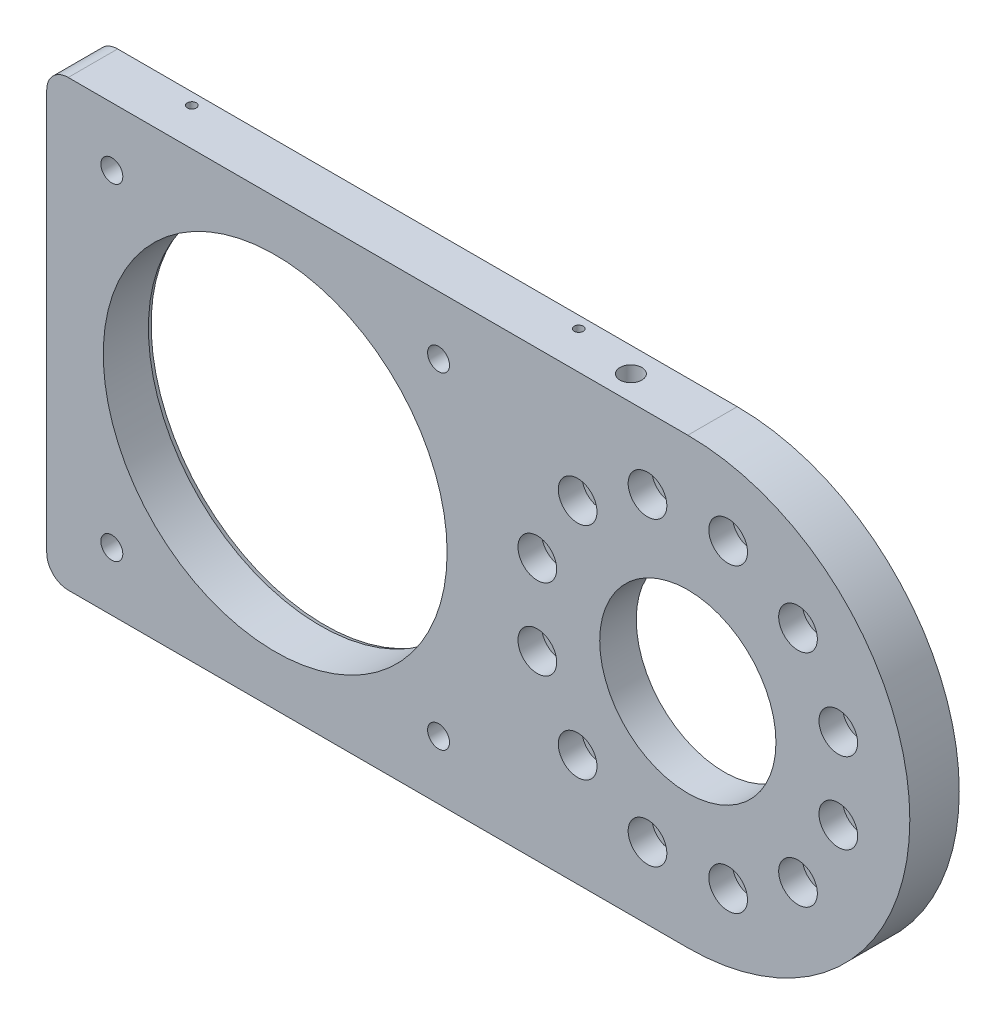
from build123d import *

# Parameters (mm, degrees)
BOSS_EXTRUDE1_DEPTH                                  = 23
FILLET1_R                                            = 10
HOLE_SIZE_PER_SOCKET_HEAD_CAP_SCREW_TYPE_D           = 11
HOLE_SIZE_PER_SOCKET_HEAD_CAP_SCREW_TYPE_CBORE_D     = 18
HOLE_SIZE_PER_SOCKET_HEAD_CAP_SCREW_TYPE_CBORE_DEPTH = 11
CIRPATTERN1_COUNT                                    = 12
SKETCH8_R                                            = 80
CUT_EXTRUDE1_DEPTH                                   = 23
SKETCH13_R                                           = 41
CUT_EXTRUDE3_DEPTH                                   = 23
SKETCH14_R                                           = 57.5
CUT_EXTRUDE4_DEPTH                                   = 6
M12_TAPPED_HOLE2_D                                   = 10.2
M5_TAPPED_HOLE1_AT_2_COUNT                           = 2
M5_TAPPED_HOLE1_AT_2_PITCH                           = 180
CHAMFER3_SIZE                                        = 2
CHAMFER3_SIZE2                                       = 0.727940469
CHAMFER4_SIZE                                        = 2
CHAMFER4_SIZE2                                       = 0.727940469
M5_TAPPED_HOLE3_D                                    = 4.2
M5_TAPPED_HOLE3_DEPTH                                = 12.4
M5_TAPPED_HOLE3_TIP                                  = 1.2618073


with BuildPart() as part:
    # Sketch1 → Boss-Extrude1 (new body)
    with BuildSketch(Plane.XY):
        with BuildLine():
            Line((0, 0), (298.3, 0))
            ThreePointArc((298.3, 0), (401.6, 103.3), (298.3, 206.6))
            Line((298.3, 206.6), (0, 206.6))
            Line((0, 206.6), (0, 0))
        make_face()
    extrude(amount=BOSS_EXTRUDE1_DEPTH)

    # Fillet1
    fillet1_edges = [part.edges().sort_by_distance(p)[0] for p in [
        (0, 206.6, 11.5),
        (0, 0, 11.5),
    ]]
    fillet(fillet1_edges, radius=FILLET1_R)

    # Hole Size per Socket Head Cap Screw Type3 (through all)
    with Locations(Plane.XY.offset(23)):
        with Locations((368.329622406, 84.53561923)):
            hole_size_per_socket_head_cap_screw_type = CounterBoreHole(HOLE_SIZE_PER_SOCKET_HEAD_CAP_SCREW_TYPE_D / 2, HOLE_SIZE_PER_SOCKET_HEAD_CAP_SCREW_TYPE_CBORE_D / 2, HOLE_SIZE_PER_SOCKET_HEAD_CAP_SCREW_TYPE_CBORE_DEPTH)

    # CirPattern1: Hole Size per Socket Head Cap Screw Type3 ×12 about axis
    cirpattern1_axis = Axis((298.3, 103.3, 0), (0, 0, 1))
    for i in range(1, CIRPATTERN1_COUNT):
        add(hole_size_per_socket_head_cap_screw_type.rotate(cirpattern1_axis, i * 360 / CIRPATTERN1_COUNT), mode=Mode.SUBTRACT)

    # Sketch8 → Cut-Extrude1 (cut)
    with BuildSketch(Plane.XY.offset(23)):
        with Locations((106.3, 103.3)):
            Circle(SKETCH8_R)
    extrude(amount=-CUT_EXTRUDE1_DEPTH, mode=Mode.SUBTRACT)

    # Sketch13 → Cut-Extrude3 (cut)
    with BuildSketch(Plane(origin=(0, 0, 0), x_dir=(-1, 0, 0), z_dir=(0, 0, -1))):
        with Locations((-298.3, 103.3)):
            Circle(SKETCH13_R)
    extrude(amount=-CUT_EXTRUDE3_DEPTH, mode=Mode.SUBTRACT)

    # Sketch14 → Cut-Extrude4 (cut)
    with BuildSketch(Plane(origin=(0, 0, 0), x_dir=(-1, 0, 0), z_dir=(0, 0, -1))):
        with Locations((-298.3, 103.3)):
            Circle(SKETCH14_R)
    extrude(amount=-CUT_EXTRUDE4_DEPTH, mode=Mode.SUBTRACT)

    # M12 Tapped Hole2 (through all)
    with Locations(Plane(origin=(0, 0, 0), x_dir=(-1, 0, 0), z_dir=(0, 0, -1))):
        with Locations((-30.286021022, 27.286021022), (-182.313978978, 27.286021022), (-30.286021022, 179.313978978), (-182.313978978, 179.313978978), (-106.3, 103.3)):
            Hole(M12_TAPPED_HOLE2_D / 2)

    # Sketch18 → M5 Tapped Hole1 (revolve, cut)
    with BuildSketch(Plane(origin=(50, 206.6, 5.5), x_dir=(0, 0, 1), z_dir=(1, 0, 0))):
        Polygon((0, 0), (0, 13.6618073), (2.1, 12.4), (2.1, 0), align=None)
    m5_tapped_hole1 = revolve(axis=Axis((50, 212.95, 5.5), (0, -1, 0)), mode=Mode.SUBTRACT)

    # M5 Tapped Hole1 at 2: M5 Tapped Hole1 ×2
    with Locations(*[(i * M5_TAPPED_HOLE1_AT_2_PITCH, 0, 0) for i in range(1, M5_TAPPED_HOLE1_AT_2_COUNT)]):
        add(m5_tapped_hole1, mode=Mode.SUBTRACT)

    # Mirror1: M5 Tapped Hole1 across plane
    add(m5_tapped_hole1.mirror(Plane.ZX.offset(103.3)), mode=Mode.SUBTRACT)

    # Mirror1 copy 1 sketch → Mirror1 copy 1 (revolve, cut)
    with BuildSketch(Plane(origin=(230, 0, 5.5), x_dir=(0, 0, 1), z_dir=(1, 0, 0))):
        Polygon((0, 0), (0, -13.6618073), (2.1, -12.4), (2.1, 0), align=None)
    revolve(axis=Axis((230, -6.35, 5.5), (0, -1, 0)), mode=Mode.SUBTRACT)

    # Chamfer3
    chamfer3_edges = [part.edges().sort_by_distance(p)[0] for p in [
        (26.3, 103.3, 0),
    ]]
    chamfer3_side = [part.faces().sort_by_distance(p)[0] for p in [
        (26.3, 103.3, 11.5),
    ]]
    chamfer(chamfer3_edges, length=CHAMFER3_SIZE, length2=CHAMFER3_SIZE2, reference=chamfer3_side[0])

    # Chamfer4
    chamfer4_edges = [part.edges().sort_by_distance(p)[0] for p in [
        (355.8, 103.3, 0),
    ]]
    chamfer4_side = [part.faces().sort_by_distance(p)[0] for p in [
        (355.8, 103.3, 3),
    ]]
    chamfer(chamfer4_edges, length=CHAMFER4_SIZE, length2=CHAMFER4_SIZE2, reference=chamfer4_side[0])

    # Sketch44 → M12 Tapped Hole3 (revolve, cut)
    with BuildSketch(Plane(origin=(260.3, 0, 11.5), x_dir=(0, 0, -1), z_dir=(1, 0, 0))):
        Polygon((0, 0), (0, 30.314389157), (5.1, 27.25), (5.1, 0), align=None)
    m12_tapped_hole3 = revolve(axis=Axis((260.3, -6.35, 11.5), (0, 1, 0)), mode=Mode.SUBTRACT)

    # Mirror5: M12 Tapped Hole3 across plane
    add(m12_tapped_hole3.mirror(Plane(origin=(0, 103.3, 0), x_dir=(0, 0, 1), z_dir=(0, -1, 0))), mode=Mode.SUBTRACT)

    # M5 Tapped Hole3
    with Locations(Plane.ZY):
        with Locations((5.5, 103.3)):
            Hole(M5_TAPPED_HOLE3_D / 2, depth=M5_TAPPED_HOLE3_DEPTH)
            with Locations((0, 0, -(M5_TAPPED_HOLE3_DEPTH + M5_TAPPED_HOLE3_TIP / 2))):  # 118° drill point
                Cone(0, M5_TAPPED_HOLE3_D / 2, M5_TAPPED_HOLE3_TIP, mode=Mode.SUBTRACT)


solid = part.part
